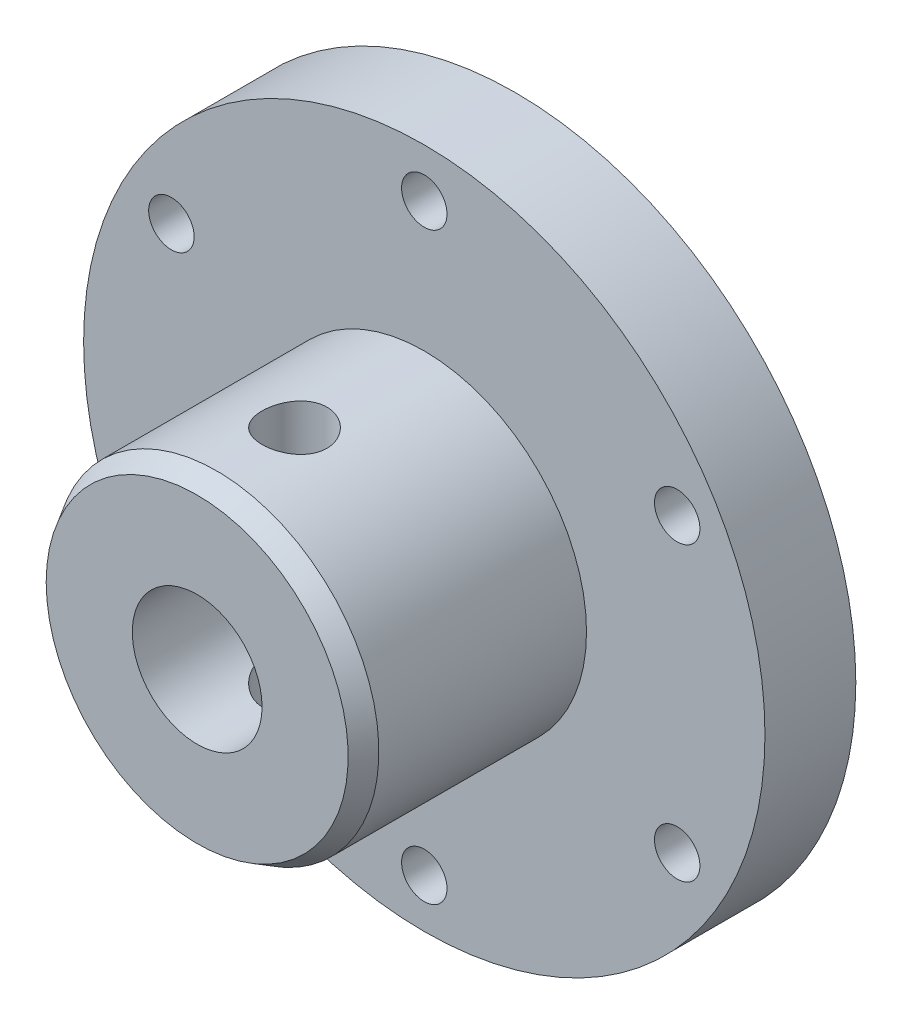
from build123d import *

# Parameters (mm, degrees)
SKETCH1_R               = 52.5
SKETCH1_R_2             = 3.5
BOSS_EXTRUDE1_DEPTH     = 14
SKETCH2_R               = 25
SKETCH2_R_2             = 10
BOSS_EXTRUDE2_DEPTH     = 35
CUT_EXTRUDE1_DEPTH      = 89.95785519
CUT_EXTRUDE1_DEPTH_BACK = 89.95785519
SKETCH3_R               = 5
CHAMFER1_SIZE           = 3
CHAMFER1_SIZE2          = 1.732050808


with BuildPart() as part:
    # Sketch1 → Boss-Extrude1 (new body)
    with BuildSketch(Plane.XY):
        Circle(SKETCH1_R)
        with Locations((0, 45)):
            Circle(SKETCH1_R_2, mode=Mode.SUBTRACT)
        with Locations((38.97114317, 22.5)):
            Circle(SKETCH1_R_2, mode=Mode.SUBTRACT)
        with Locations((38.97114317, -22.5)):
            Circle(SKETCH1_R_2, mode=Mode.SUBTRACT)
        with Locations((0, -45)):
            Circle(SKETCH1_R_2, mode=Mode.SUBTRACT)
        with Locations((-38.97114317, -22.5)):
            Circle(SKETCH1_R_2, mode=Mode.SUBTRACT)
        with Locations((-38.97114317, 22.5)):
            Circle(SKETCH1_R_2, mode=Mode.SUBTRACT)
    extrude(amount=BOSS_EXTRUDE1_DEPTH)

    # Sketch2 → Boss-Extrude2 (add)
    with BuildSketch(Plane.XY.offset(14)):
        Circle(SKETCH2_R)
        Circle(SKETCH2_R_2, mode=Mode.SUBTRACT)
    extrude(amount=BOSS_EXTRUDE2_DEPTH)

    # Sketch3 → Cut-Extrude1 (cut, two sides: drawn at the far end of the back side and taken through both)
    with BuildSketch(Plane(origin=(0, 0, 0), x_dir=(1, 0, 0), z_dir=(0, 1, 0)).offset(-CUT_EXTRUDE1_DEPTH_BACK)):
        with Locations(Location((0, -34, 0), (0, 0, 270))):
            Circle(SKETCH3_R)
    extrude(amount=CUT_EXTRUDE1_DEPTH + CUT_EXTRUDE1_DEPTH_BACK, mode=Mode.SUBTRACT)

    # Chamfer1
    chamfer1_edges = [part.edges().sort_by_distance(p)[0] for p in [
        (-25, 0, 49),
    ]]
    chamfer1_side = [part.faces().sort_by_distance(p)[0] for p in [
        (-25, 0, 31.5),
    ]]
    chamfer(chamfer1_edges, length=CHAMFER1_SIZE, length2=CHAMFER1_SIZE2, reference=chamfer1_side[0])


solid = part.part
